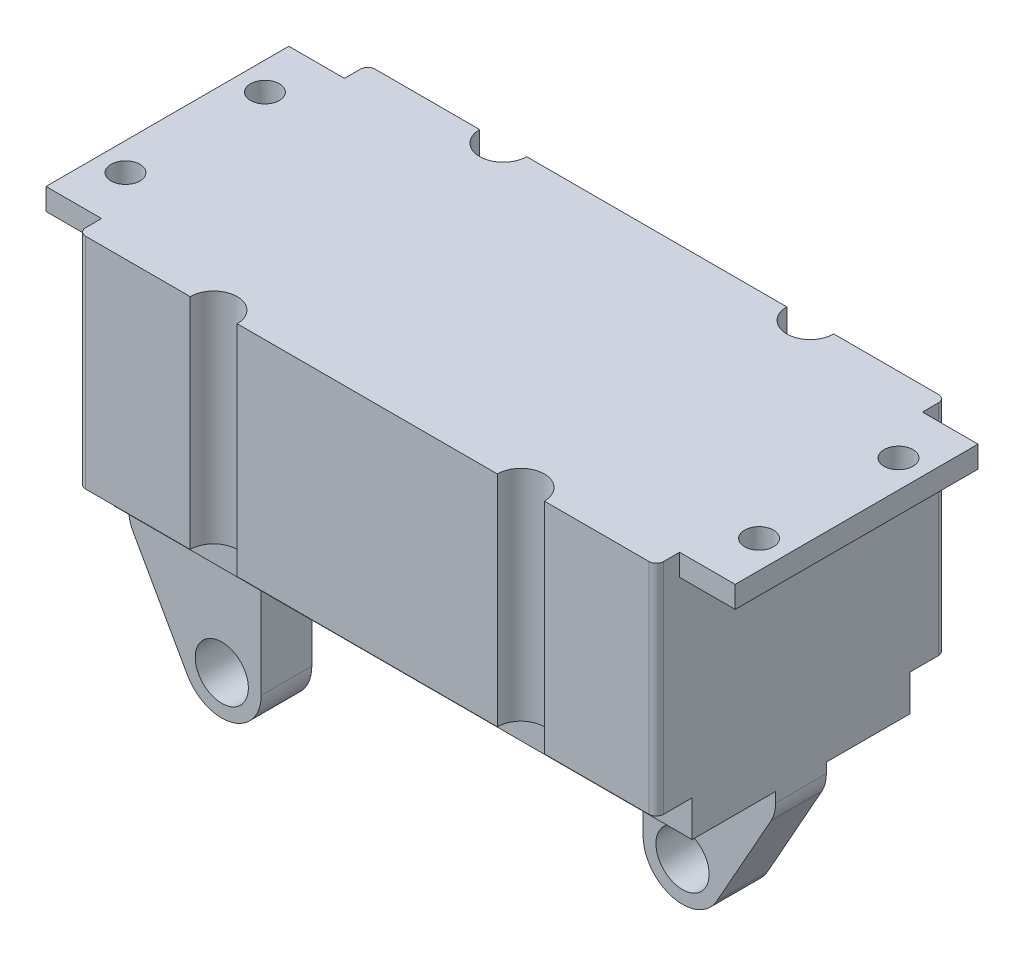
SolidWorks part; units mm, degrees
ref_plane "Front Plane" through (0, 0, 0) normal (0, 0, 1) x (1, 0, 0)
ref_plane "Top Plane" through (0, 0, 0) normal (0, 1, 0) x (1, 0, 0)
ref_plane "Right Plane" through (0, 0, 0) normal (1, 0, 0) x (0, 0, -1)
other "Configuration Table"
sketch "Sketch1" plane through (0, 0, 0) normal (0, 0, 1) x (1, 0, 0)
  line L1 (-39.9424, 66.0721) -> (39.9424, 66.0721)
  line L2 (-39.9424, 66.0721) -> (-39.9424, 35.8074)
  line L3 (-39.9424, 35.8074) -> (39.9424, 35.8074)
  line L4 (39.9424, 66.0721) -> (39.9424, 35.8074)
  line L5 (-39.9424, 66.0721) -> (39.9424, 35.8074) construction
  line L6 (-39.9424, 35.8074) -> (39.9424, 66.0721) construction
  point P0 (0, 50.9397)
extrude "Boss-Extrude1" add sketch "Sketch1" along normal mid plane 40
sketch "Sketch2" plane through (0, 35.8074, 0) normal (0, -1, 0) x (1, 0, 0)
  line L0 (39.9424, 20) -> (39.9424, -20) construction
  line L1 (-39.9424, 15.0442) -> (39.9424, 15.0442)
  line L2 (-39.9424, 15.0442) -> (-39.9424, -15.0442)
  line L3 (-39.9424, -15.0442) -> (39.9424, -15.0442)
  line L4 (39.9424, 15.0442) -> (39.9424, -15.0442)
  line L5 (-39.9424, 15.0442) -> (39.9424, -15.0442) construction
  line L6 (-39.9424, -15.0442) -> (39.9424, 15.0442) construction
  point P0 (0, 0)
extrude "Boss-Extrude2" add sketch "Sketch2" along normal blind 5
sketch "Sketch3" plane through (0, 66.0721, 0) normal (0, 1, 0) x (1, 0, 0)
  line L0 (39.9424, 20) -> (-39.9424, 20) construction
  line L1 (0, 0) -> (0, 20) construction
  line L2 (0, 0) -> (-39.4159, 0) construction
  circle A0 centre (-21.2239, 20) radius 3.2458
  circle A1 centre (21.2239, 20) radius 3.2458
  circle A2 centre (21.2239, -20) radius 3.2458
  circle A3 centre (-21.2239, -20) radius 3.2458
extrude "Cut-Extrude1" cut sketch "Sketch3" against normal blind 47
fillet "Fillet1" radius 1 4 edges at (-39.9424, 50.9397, -20) (39.9424, 50.9397, -20) (39.9424, 50.9397, 20) (-39.9424, 50.9397, 20)
ref_plane "Plane1" through (0, 0, 13.0442) normal (0, 0, 1) x (1, 0, 0)
sketch "Sketch4" plane through (0, 0, 13.0442) normal (0, 0, 1) x (1, 0, 0)
  line L0 (-39.9424, 30.8074) -> (-39.9424, 29.4277)
  line L2 (-21.6207, 30.8074) -> (-21.6207, 16.2887)
  line L3 (39.9424, 30.8074) -> (-39.9424, 30.8074) construction
  line L4 (-39.9424, 30.8074) -> (-39.9424, 35.8074) construction
  line L5 (-39.3037, 26.9825) -> (-31.8151, 13.6259)
  line L6 (-39.9424, 30.8074) -> (-21.6207, 30.8074)
  arc A0 (-31.8151, 13.6259) -> (-21.6207, 16.2887) centre (-27.0657, 16.2887) ccw
  arc A1 (-39.9424, 29.4277) -> (-39.3037, 26.9825) centre (-34.9424, 29.4277) ccw
  circle A2 centre (-27.0657, 16.2887) radius 3.6746
  dimension "D1" = 5
extrude "Boss-Extrude3" add sketch "Sketch4" against normal blind 7
mirror "Mirror1" about plane through (0, 0, 0) normal (0, 0, 1) of "Boss-Extrude3"
sketch "Sketch5" plane through (0, 0, 0) normal (0, 0, 1) x (1, 0, 0)
  line L0 (0, 30.8074) -> (0, 0) construction
  line L1 (39.9424, 30.8074) -> (-39.9424, 30.8074) construction
  line L2 (21.6207, 16.2887) -> (21.6207, 30.8074)
  line L3 (39.3037, 26.9825) -> (31.8151, 13.6259)
  line L12 (39.9424, 30.8074) -> (39.9424, 29.4277)
  line L13 (21.6207, 30.8074) -> (39.9424, 30.8074)
  arc A0 (31.8151, 13.6259) -> (21.6207, 16.2887) centre (27.0657, 16.2887) cw
  arc A1 (39.9424, 29.4277) -> (39.3037, 26.9825) centre (34.9424, 29.4277) cw
  circle A7 centre (27.0657, 16.2887) radius 3.6746
extrude "Boss-Extrude4" add sketch "Sketch5" along normal mid plane 7
sketch "Sketch6" plane through (0, 66.0721, 0) normal (0, 1, 0) x (1, 0, 0)
  line L0 (-39.9424, -19) -> (-39.9424, 19) construction
  line L1 (-47.6255, 16.78) -> (-39.9424, 16.78)
  line L2 (-47.6255, 16.78) -> (-47.6255, -16.78)
  line L3 (-47.6255, -16.78) -> (-39.9424, -16.78)
  line L5 (-47.6255, 16.78) -> (-39.9424, 0) construction
  line L6 (-47.6255, -16.78) -> (-39.9424, 0) construction
  line L7 (-39.9424, 16.78) -> (-39.9424, -16.78)
  line L8 (0, 0) -> (0, 16.78) construction
  line L9 (47.6255, -16.78) -> (39.9424, 0) construction
  line L10 (47.6255, 16.78) -> (39.9424, 0) construction
  line L11 (39.9424, 16.78) -> (39.9424, -16.78)
  line L12 (47.6255, -16.78) -> (39.9424, -16.78)
  line L13 (47.6255, 16.78) -> (47.6255, -16.78)
  line L14 (47.6255, 16.78) -> (39.9424, 16.78)
  line L15 (-47.6255, 0) -> (-41.7913, 0) construction
  circle A0 centre (-43.784, 9.6351) radius 2
  circle A1 centre (-43.784, -9.6351) radius 2
  circle A2 centre (43.784, -9.6351) radius 2
  circle A3 centre (43.784, 9.6351) radius 2
  point P0 (-39.9424, 0)
  point P15 (39.9424, 0)
extrude "Boss-Extrude5" add sketch "Sketch6" against normal blind 3
